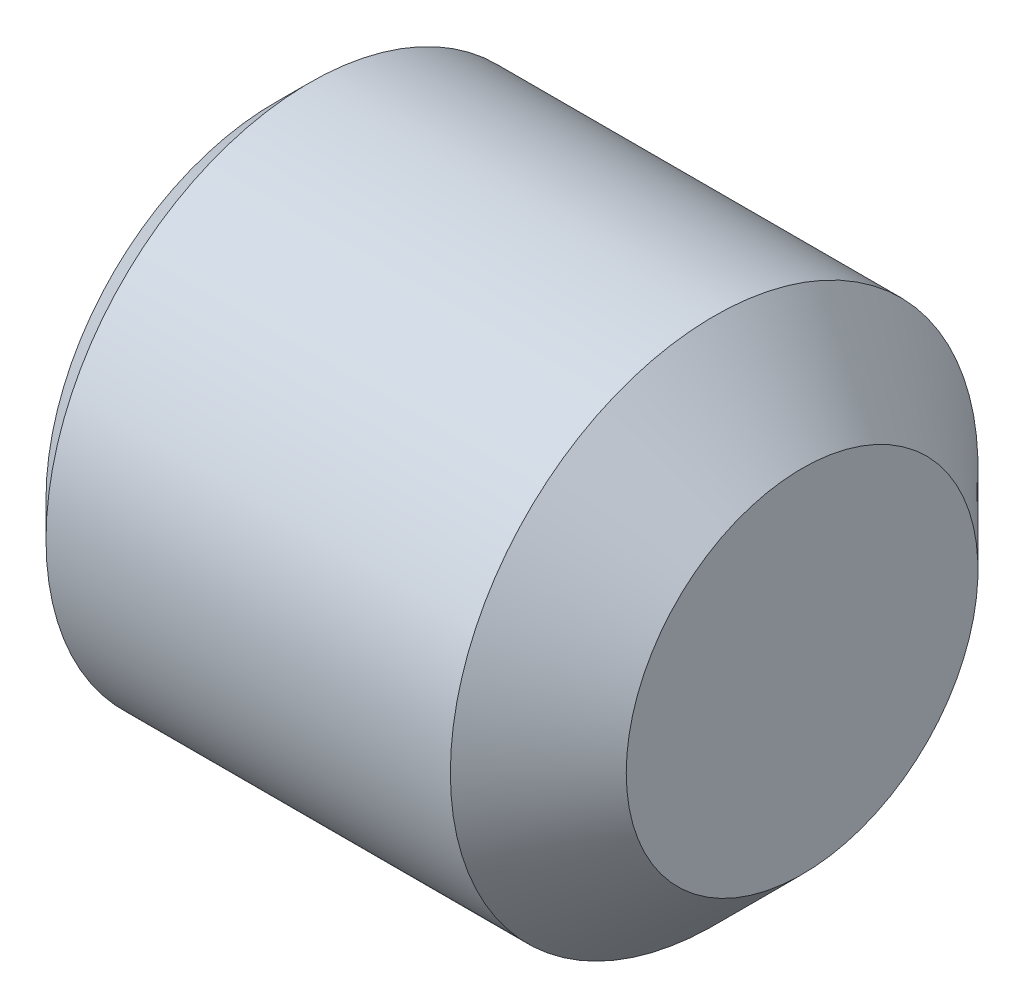
SolidWorks part; units mm, degrees
revolve "Base-Revolve" add sketch "Sketch1" angle 360 about L6
sketch "Sketch1" plane through (0, 0, 0) normal (0, 0, 1) x (1, 0, 0)
  line L0 (0, 0) -> (3, 0)
  line L1 (3, 0) -> (3, 1)
  line L2 (3, 1) -> (2.5, 1.5)
  line L3 (2.5, 1.5) -> (0.201, 1.5)
  line L4 (0.201, 1.5) -> (0, 1.299)
  line L5 (0, 1.299) -> (0, 0)
  line L6 (-0.2778, 0) -> (5.1995, 0) construction
cosmetic thread "Cosmetic Thread1" parameters "df"=2.598
extrude "Cut-Extrude1" cut sketch "Sketch2" against normal blind 1.2
sketch "Sketch2" plane through (0, 0, 0) normal (-1, 0, 0) x (0, 0, 1)
  line L1 (-0.4325, -0.7491) -> (0.4325, -0.7491)
  line L2 (0.4325, -0.7491) -> (0.865, 0)
  line L3 (0.865, 0) -> (0.4325, 0.7491)
  line L4 (0.4325, 0.7491) -> (-0.4325, 0.7491)
  line L5 (-0.4325, 0.7491) -> (-0.865, 0)
  line L6 (-0.865, 0) -> (-0.4325, -0.7491)
  circle A0 centre (0, 0) radius 0.7491 construction
material "45H级"
ref_plane "Front" through (0, 0, 0) normal (0, 0, 1) x (1, 0, 0)
ref_plane "Top" through (0, 0, 0) normal (0, 1, 0) x (1, 0, 0)
ref_plane "Right" through (0, 0, 0) normal (1, 0, 0) x (0, 0, -1)
sketch "Dimension-Sketch" plane through (0, 0, 0) normal (0, 0, 1) x (1, 0, 0)
  line L0 (0, 0) -> (3, 0)
  point P3 (1.2, 0)
  point P4 (2.5, 0)
  point P5 (1, 0)
  point P6 (2.598, 0)
  point P7 (3, 0)
  point P8 (1.27, 0)
sketch "Sketch4" plane through (0, 0, 0) normal (0, 0, 1) x (1, 0, 0)
  line L0 (-0.2778, 0) -> (1.1933, 0) construction
  line L2 (-0.2778, 0) -> (5.1995, 0) construction
  line L3 (1.2, 0.7491) -> (1.6325, 0)
  line L4 (1.6325, 0) -> (1.2, 0)
  line L5 (1.2, 0) -> (1.2, 0.7491)
  line L6 (1.2, 0.7491) -> (0, 0.7491) construction
revolve "Cut-Revolve2" cut sketch "Sketch4" angle 360 about L0
sketch "Sketch5" plane through (0, 0, 0) normal (0, 0, 1) x (1, 0, 0)
  line L0 (0.201, 1.5) -> (0.701, 1.5)
  line L1 (2.5, 1.5) -> (0.201, 1.5) construction
  line L2 (0.701, 1.5) -> (0.4483, 1.067)
  line L3 (0.4483, 1.067) -> (0.201, 1.5)
  line L5 (5.1995, 0) -> (3.6008, 0) construction
  line L6 (-0.2778, 0) -> (5.1995, 0) construction
  line L7 (0.201, 1.5) -> (0, 1.299) construction
revolve "Cut-Revolve3" [suppressed] cut sketch "Sketch5" angle 360 about L5
pattern_linear "LPattern1" [suppressed] count 6
equation "\"l@Sketch1\"=\"l@Dimension-Sketch\""
equation "\"d@Sketch1\"=\"d@Dimension-Sketch\""
equation "\"df@Sketch1\" = \"df@Dimension-Sketch\""
equation "\"dp@Sketch1\" = \"dp@Dimension-Sketch\""
equation "\"e@Sketch2\" = \"e@Dimension-Sketch\""
equation "\"t@Cut-Extrude1\" = \"t@Dimension-Sketch\""
equation "\"P@Sketch5\" = \"P@Dimension-Sketch\""
equation "\"D1@Sketch5\" = \"P@Dimension-Sketch\"*0.866"
equation "\"P@LPattern1\" = \"P@Dimension-Sketch\""
equation "\"D1@LPattern1\" = \"l@Dimension-Sketch\"/\"P@Dimension-Sketch\""
equation "\"df@Cosmetic Thread1\"=\"df@Dimension-Sketch\""
equation "\"D2@Sketch4\" = \"t@Dimension-Sketch\""
